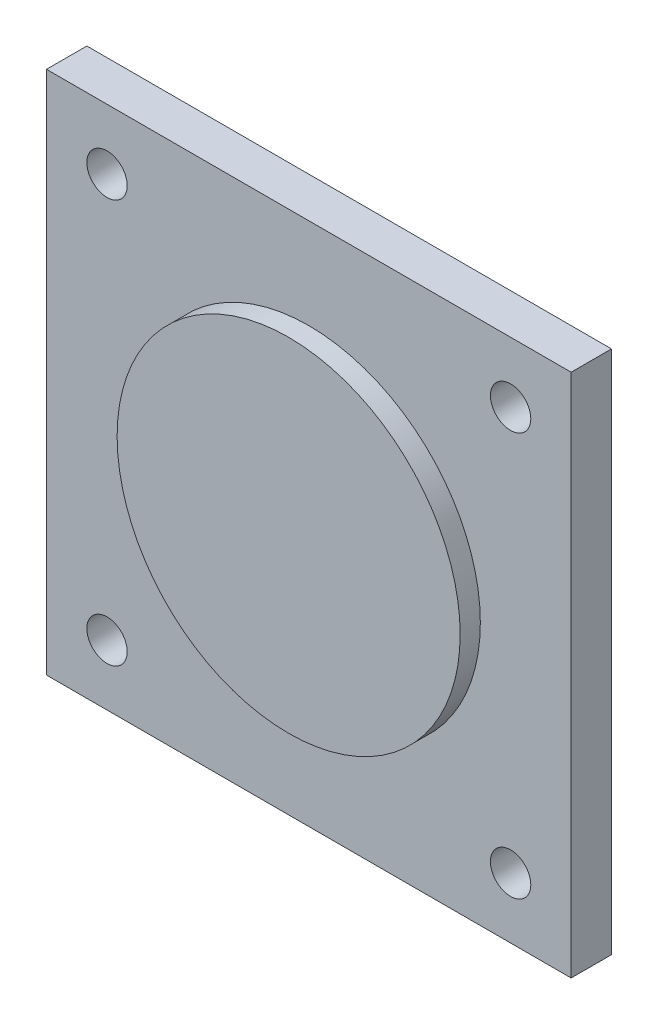
from build123d import *

# Parameters (mm, degrees)
SKETCH1_W           = 130
SKETCH1_H           = 130
BOSS_EXTRUDE1_DEPTH = 10
SKETCH2_R           = 42.5
BOSS_EXTRUDE2_DEPTH = 5
SKETCH3_R           = 5
CUT_EXTRUDE1_DEPTH  = 51


with BuildPart() as part:
    # Sketch1 → Boss-Extrude1 (new body)
    with BuildSketch(Plane.XY):
        Rectangle(SKETCH1_W, SKETCH1_H)
    extrude(amount=BOSS_EXTRUDE1_DEPTH)

    # Sketch2 → Boss-Extrude2 (add)
    with BuildSketch(Plane.XY.offset(10)):
        Circle(SKETCH2_R)
    extrude(amount=BOSS_EXTRUDE2_DEPTH)

    # Sketch3 → Cut-Extrude1 (cut)
    with BuildSketch(Plane.XY.offset(10)):
        with Locations((50, 50)):
            Circle(SKETCH3_R)
        with Locations((-50, 50)):
            Circle(SKETCH3_R)
        with Locations((-50, -50)):
            Circle(SKETCH3_R)
        with Locations((50, -50)):
            Circle(SKETCH3_R)
    extrude(amount=-CUT_EXTRUDE1_DEPTH, mode=Mode.SUBTRACT)


solid = part.part
